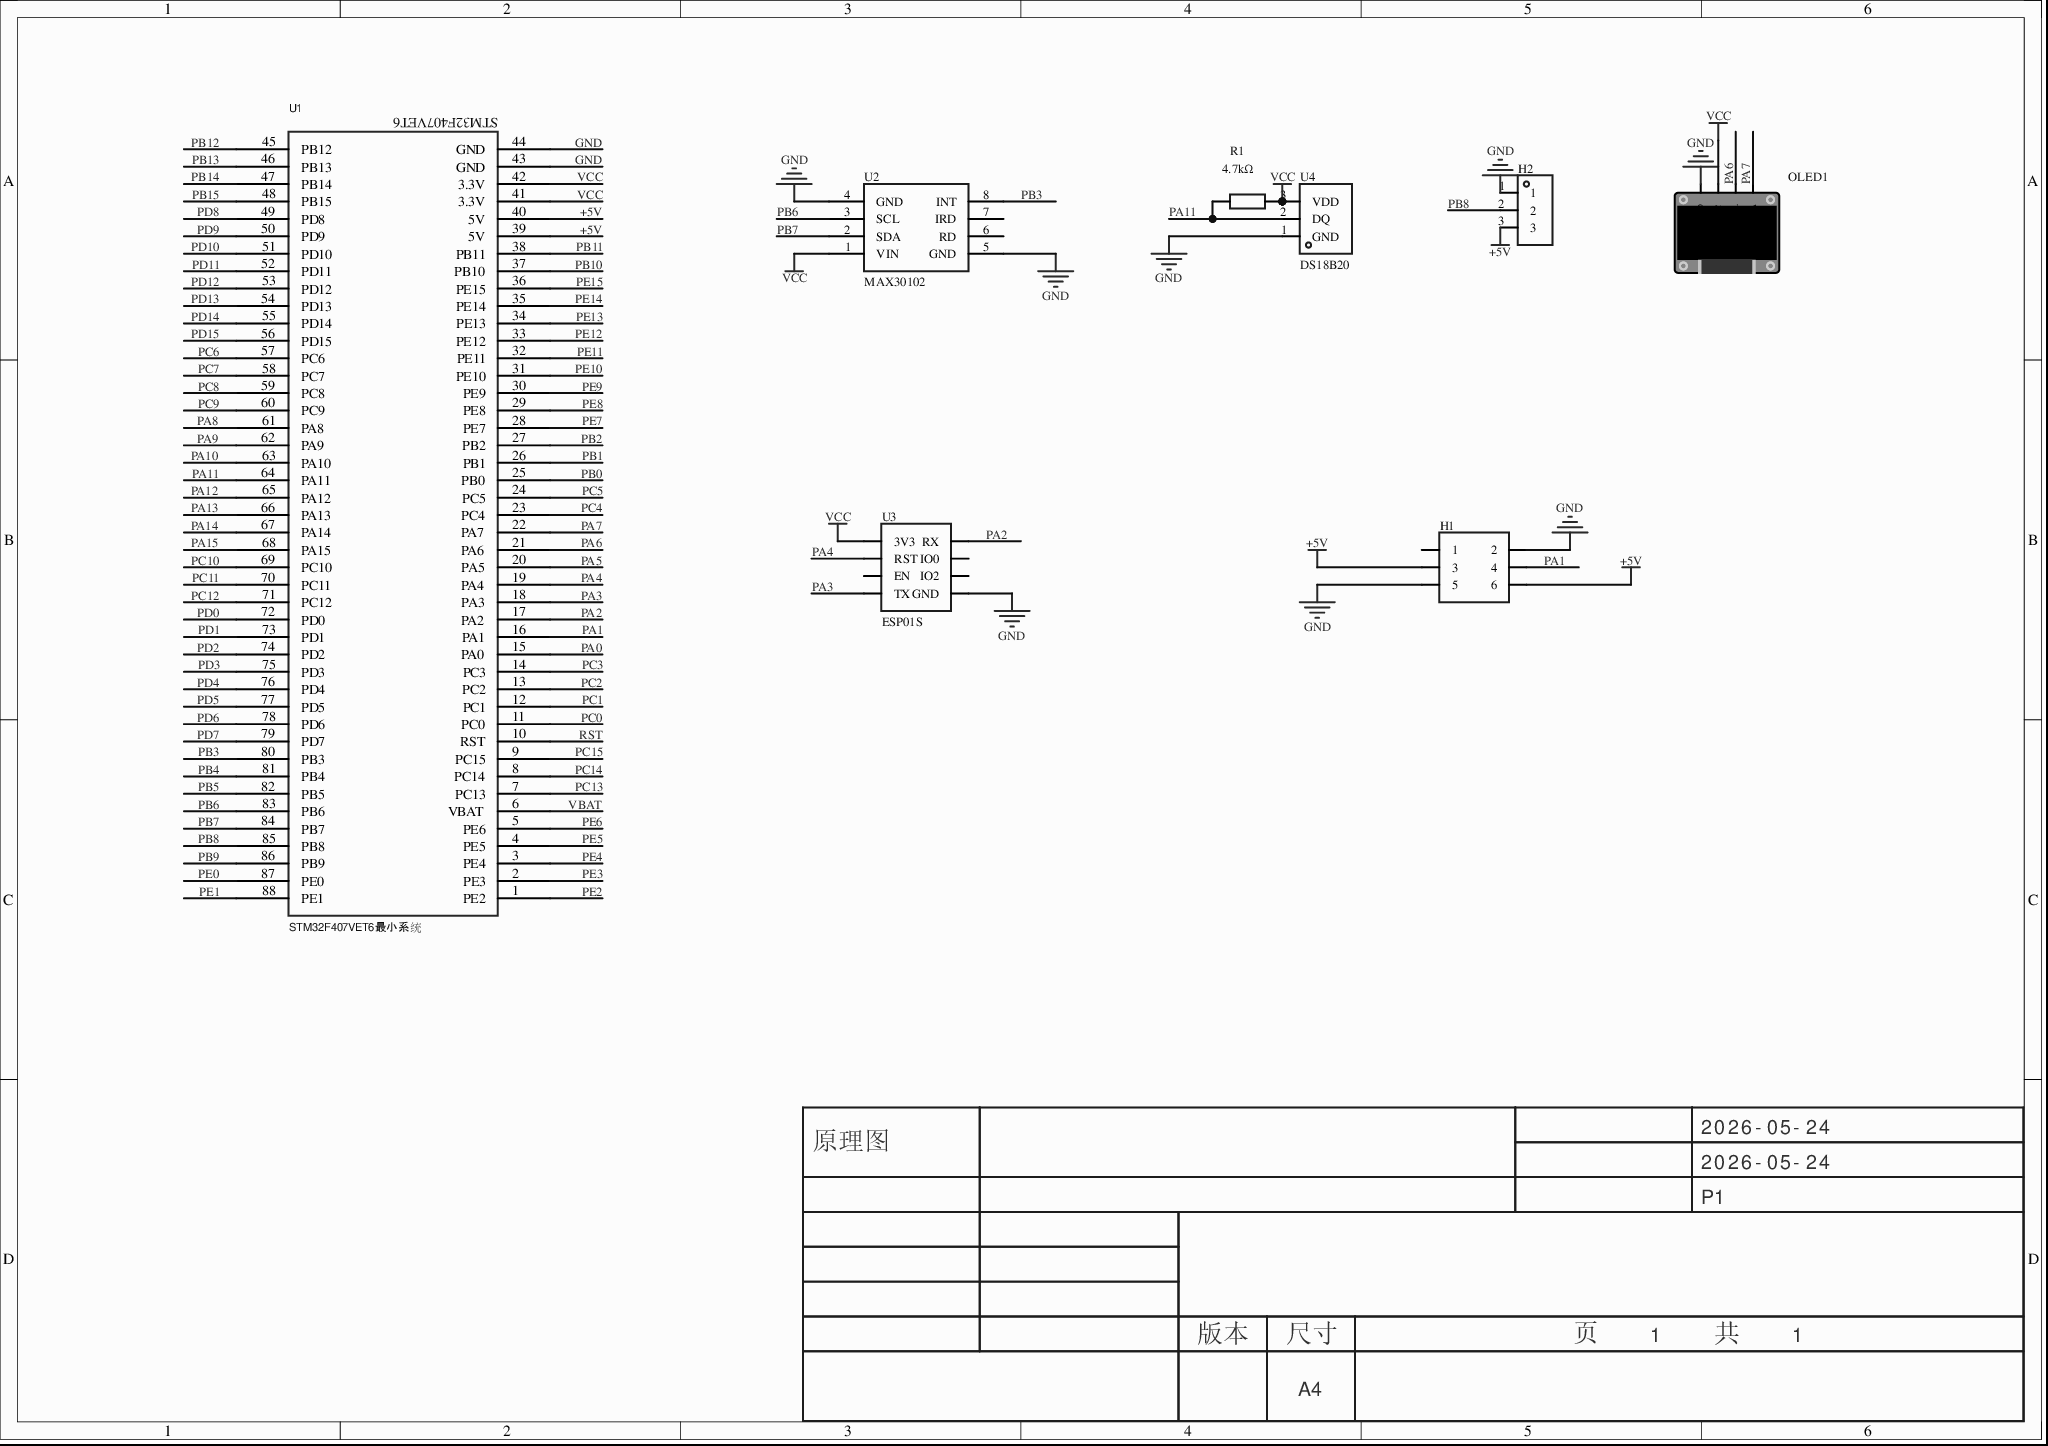
[diagram p0: MISC51903-3.schdoc]
# Altium project MISC51903-2.PrjPcb
1 sheet, 8 parts. Net scope: global (net labels, ports and power ports of the same name join across sheets).
Board file: MISC51903.pcbdoc

## Sheet MISC51903-3.schdoc
size 297 x 209 mm; Version: V1.0; @Project Name: MISC51903; @Update Date: 2026-05-24; @Create Date: 2026-05-24; @Board Name: MISC51903; @Create Time: 11:44:03; @Page Count: 1; @Page No: 1; @Schematic Name: MISC51903; @Update Time: 11:44:03; Size: A4

### Parts
H1  (no value)  [HDR-TH_6P-P2.54-V-F-R2-C3-S2.54]
H2  (no value)  [HDR-TH_3P-P2.54-V-F]
OLED1  (no value)  [0.96OLED_4P]
R1  4.7kΩ  [Res_1/8W]
U1  STM32F407VET6最小系统  [STM32F407VET6最小系统]
U2  MAX30102  [MAX30102]
U3  ESP01S  [ESP01S]
U4  DS18B20  [TO-92-3_L4.5-W3.5-P1.27-L]

### Nets
+5V: H1.3 H1.6 H2.3 U1.39(5V) U1.40(5V)
GND: H1.2 H1.5 H2.1 OLED1.1(GND) U1.43(GND) U1.44(GND) U2.4(GND) U2.5(GND) U3.5(GND) U4.1(GND)
VCC: OLED1.2(VCC) R1.2 U1.41(3.3V) U1.42(3.3V) U2.1(VIN) U3.1(3V3) U4.3(VDD)
PA0: U1.15(PA0)
PA1: H1.4 U1.16(PA1)
PA2: U1.17(PA2) U3.8(RX)
PA3: U1.18(PA3) U3.4(TX)
PA4: U1.19(PA4) U3.2(RST)
PA5: U1.20(PA5)
PA6: OLED1.3(SCL) U1.21(PA6)
PA7: OLED1.4(SDA) U1.22(PA7)
PA8: U1.61(PA8)
PA9: U1.62(PA9)
PA10: U1.63(PA10)
PA11: R1.1 U1.64(PA11) U4.2(DQ)
PA12: U1.65(PA12)
PA13: U1.66(PA13)
PA14: U1.67(PA14)
PA15: U1.68(PA15)
PB0: U1.25(PB0)
PB1: U1.26(PB1)
PB2: U1.27(PB2)
PB3: U1.80(PB3) U2.8(INT)
PB4: U1.81(PB4)
PB5: U1.82(PB5)
PB6: U1.83(PB6) U2.3(SCL)
PB7: U1.84(PB7) U2.2(SDA)
PB8: H2.2 U1.85(PB8)
PB9: U1.86(PB9)
PB10: U1.37(PB10)
PB11: U1.38(PB11)
PB12: U1.45(PB12)
PB13: U1.46(PB13)
PB14: U1.47(PB14)
PB15: U1.48(PB15)
PC0: U1.11(PC0)
PC1: U1.12(PC1)
PC2: U1.13(PC2)
PC3: U1.14(PC3)
PC4: U1.23(PC4)
PC5: U1.24(PC5)
PC6: U1.57(PC6)
PC7: U1.58(PC7)
PC8: U1.59(PC8)
PC9: U1.60(PC9)
PC10: U1.69(PC10)
PC11: U1.70(PC11)
PC12: U1.71(PC12)
PC13: U1.7(PC13)
PC14: U1.8(PC14)
PC15: U1.9(PC15)
PD0: U1.72(PD0)
PD1: U1.73(PD1)
PD2: U1.74(PD2)
PD3: U1.75(PD3)
PD4: U1.76(PD4)
PD5: U1.77(PD5)
PD6: U1.78(PD6)
PD7: U1.79(PD7)
PD8: U1.49(PD8)
PD9: U1.50(PD9)
PD10: U1.51(PD10)
PD11: U1.52(PD11)
PD12: U1.53(PD12)
PD13: U1.54(PD13)
PD14: U1.55(PD14)
PD15: U1.56(PD15)
PE0: U1.87(PE0)
PE1: U1.88(PE1)
PE2: U1.1(PE2)
PE3: U1.2(PE3)
PE4: U1.3(PE4)
PE5: U1.4(PE5)
PE6: U1.5(PE6)
PE7: U1.28(PE7)
PE8: U1.29(PE8)
PE9: U1.30(PE9)
PE10: U1.31(PE10)
PE11: U1.32(PE11)
PE12: U1.33(PE12)
PE13: U1.34(PE13)
PE14: U1.35(PE14)
PE15: U1.36(PE15)
RST: U1.10(RST)
VBAT: U1.6(VBAT)

Not connected (* = marked no-connect by the designer): H1 1; U2 6(RD) 7(IRD); U3 3(EN) 6(IO2) 7(IO0)

### Notes on the sheet
- 2026-05-24
- 原理图
- P1
- 版本
- 尺寸
- A4
- 页    1    共    1

### Library data of the parts
H1 = HDR-F_2.54_2x3: Symbol: HDR-F-2.54_2x3; ConvertToPcb: yes; ModelId: 6dbaf143e10146ae9674d03402f6f9fb0819f05c4eef4c71ace90d822a990e87; ModelName: HDR-TH_6P-P2.54-F-LI-2X3P; ModelTransform: 315.7474,196.85,0,0,0,0,0,0,-125.984; Device: HDR-F_2.54_2x3; AddInBom: yes; SupplierPart: C92272; Supplier Footprint: 插件; FootprintName: HDR-TH_6P-P2.54-V-F-R2-C3-S2.54
H2 = HDR-F_2.54_1x3P: Symbol: PM254V-11-03-H85; ConvertToPcb: yes; ModelId: f3b3cc5aae9641bf9e56fc160cef875b0819f05c4eef4c71ace90d822a990e87; ModelName: HDR2.54-F-LI-1X3P; ModelTransform: 299.9994,100,0,0,0,0,0,0,-118.11; Device: HDR-F_2.54_1x3P; AddInBom: yes; SupplierPart: C541850; Supplier Footprint: 插件; FootprintName: HDR-TH_3P-P2.54-V-F
OLED1 = 0.96OLED模块_4P: ConvertToPcb: yes; ModelId: 79c000fdb68d45a296c2e9bedf4f90550819f05c4eef4c71ace90d822a990e87; ModelTransform: 1393.69792,1318.895,0,0,0,0,0,-560.079,-137.795; Symbol: 0.96OLED模块_4P; Device: 0.96OLED模块_4P; AddInBom: yes; FootprintName: 0.96OLED_4P; Supplier Footprint: 插件; ModelName: 0.96OLED_4P
R1 = Res_AXIAL-1/8W: Symbol: 电阻; ConvertToPcb: yes; ModelId: b2b5ae7ae4c642178fe0039925c86a3f0819f05c4eef4c71ace90d822a990e87; ModelName: RES-TH_BD1.8-L3.2-P7.20-D0.4; ModelTransform: 282.86,66.88,253.09,0,0,0,0,0,-191; Device: Res_AXIAL-1/8W; Value: 4.7kΩ; AddInBom: yes; Supplier Footprint: 轴向引线; FootprintName: Res_1/8W
U2 = MAX30102: AddInBom: yes; ModelTransform: 0, 0, 0, 0, 0, 0, 0, 0, 0; Symbol: MAX30102; Device: MAX30102; ConvertToPcb: yes; FootprintName: MAX30102
U3 = ESP01S: ConvertToPcb: yes; Symbol: ESP01S; Device: ESP01S; AddInBom: yes; FootprintName: ESP01S
U4 = DS18B20: 检测温度:-55℃~+125℃;精度:±0.4℃;接口类型:单总线;; Manufacturer: HXY MOSFET(华轩阳电子); Symbol: DS18B20_C5451632; AddInBom: yes; ModelId: 45fa6cddef3743c6aacf8db740a3bc4c0819f05c4eef4c71ace90d822a990e87; ModelTransform: 177.165,137.795,0,0,0,0,0,29.528,-98.425; Tolerance: ±0.4℃; Voltage - Supply: 2.5V~5.5V; Standby Current: 1uA; Interface: 单总线; Temperature Conversion Time: 400ms; Temperature Resolution: 12bit; Device: DS18B20; LCSC Part Name: 温度-10℃~70℃ 精度±0.4℃ 电压2.5V~5.5V; SupplierPart: C5451632; ManufacturerPart: DS18B20; Supplier Footprint: TO-92; JLCPCB Part Class: Extended Part; Datasheet: https://item.szlcsc.com/datasheet/DS18B20/6355375.html; Supplier: LCSC; ConvertToPcb: yes; FootprintName: TO-92-3_L4.5-W3.5-P1.27-L; ModelName: TO-92-3_L4.5-W3.5-P1.27-L; Detection Temperature Range: -55℃~+125℃; Operating Temperature: -
U1 = STM32F407VET6最小系统: Symbol: STM32F407VET6最小系统; Device: STM32F407VET6最小系统; FootprintName: STM32F407VET6最小系统